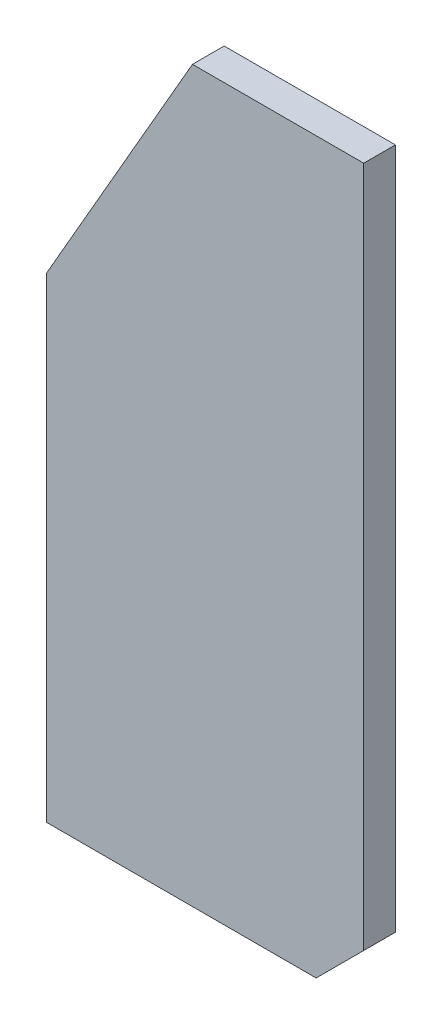
SolidWorks part; units mm, degrees
material "XRAAT"
ref_plane "前视基准面" through (0, 0, 0) normal (0, 0, 1) x (1, 0, 0)
ref_plane "上视基准面" through (0, 0, 0) normal (0, 1, 0) x (1, 0, 0)
ref_plane "右视基准面" through (0, 0, 0) normal (1, 0, 0) x (0, 0, -1)
sketch "草图1" plane through (0, 0, 0) normal (0, 0, 1) x (1, 0, 0)
  line L0 (0, 0) -> (0, 150)
  line L1 (0, 150) -> (46, 230)
  line L2 (46, 230) -> (100, 230)
  line L3 (100, 230) -> (100, 0)
  line L4 (100, 0) -> (0, 0)
  dimension "D1" = 100
  dimension "D2" = 150
  dimension "D3" = 230
  dimension "D4" = 54
extrude "凸台-拉伸1" add sketch "草图1" along normal mid plane 10
chamfer "倒角1" distance 15 angle 45 1 edges at (100, 0, 0)
